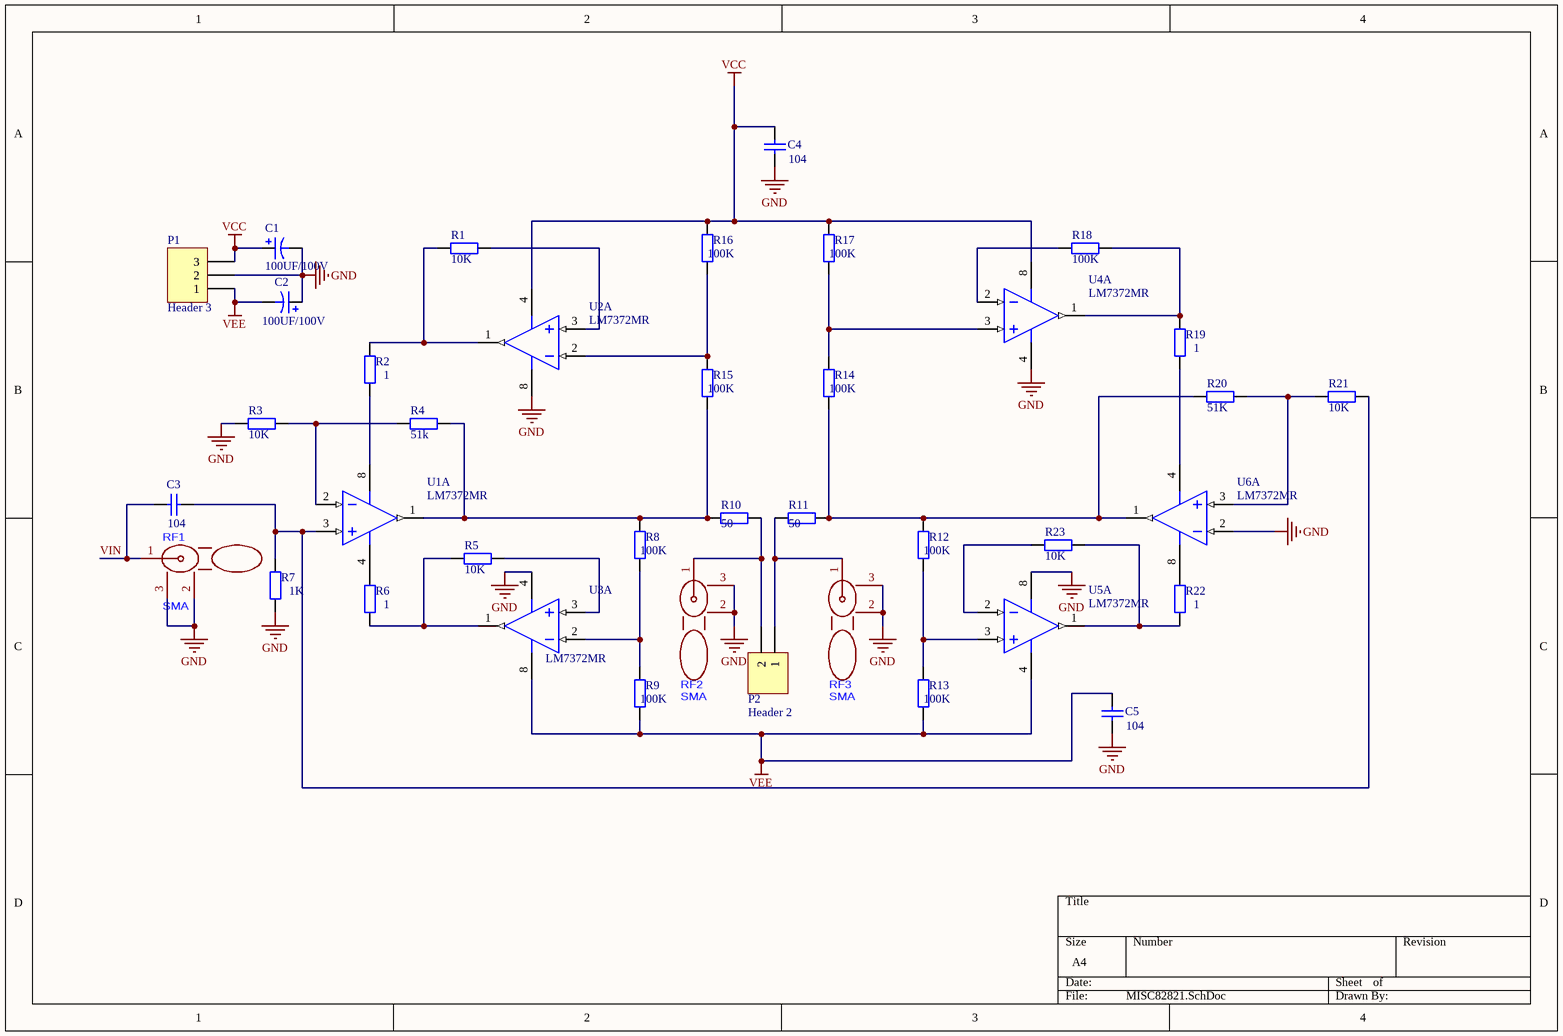
[diagram p0: MISC82821.SchDoc]
# Altium project MISC82821-15.PrjPcb
1 sheet, 39 parts. Net scope: global (net labels, ports and power ports of the same name join across sheets).
Board file: MISC82821.PcbDoc

## Sheet MISC82821.SchDoc
size A4

### Parts
C1  100UF/100V  [C0805]
C2  100UF/100V  [C0805]
C3  104  [C1206]
C4  104  [C1206]
C5  104  [C1206]
P1  Header 3  [HDR1X3]
P2  Header 2  [HDR1X2]
R1  10K  [AXIAL-0.4]
R2  1  [AXIAL-0.4]
R3  10K  [AXIAL-0.4]
R4  51k  [AXIAL-0.4]
R5  10K  [AXIAL-0.4]
R6  1  [AXIAL-0.4]
R7  1K  [AXIAL-0.4]
R8  100K  [AXIAL-0.4]
R9  100K  [AXIAL-0.4]
R10  50  [AXIAL-0.4]
R11  50  [AXIAL-0.4]
R12  100K  [AXIAL-0.4]
R13  100K  [AXIAL-0.4]
R14  100K  [AXIAL-0.4]
R15  100K  [AXIAL-0.4]
R16  100K  [AXIAL-0.4]
R17  100K  [AXIAL-0.4]
R18  100K  [AXIAL-0.4]
R19  1  [AXIAL-0.4]
R20  51K  [AXIAL-0.4]
R21  10K  [AXIAL-0.4]
R22  1  [AXIAL-0.4]
R23  10K  [AXIAL-0.4]
RF1  SMA  [SMA-SMD_HJ-SMA313]
RF2  SMA  [SMA-SMD_HJ-SMA313]
RF3  SMA  [SMA-SMD_HJ-SMA313]
U1  LM7372MR  [MRA08B_N]  (part A of 3)
U2  LM7372MR  [MRA08B_N]  (part A of 3)
U3  LM7372MR  [MRA08B_N]  (part A of 3)
U4  LM7372MR  [MRA08B_N]  (part A of 3)
U5  LM7372MR  [MRA08B_N]  (part A of 3)
U6  LM7372MR  [MRA08B_N]  (part A of 3)

### Nets
GND: C1.2 C2.1 C4.1 C5.1 P1.2 R3.1 R7.1 RF1.2 RF1.3 RF2.2 RF2.3 RF3.2 RF3.3 U2.8(V+) U3.4(V-) U4.4(V-) U5.8(V+) U6.2(INA-)
VCC: C1.1 C4.2 P1.3 R16.2 R17.2 U2.4(V-) U4.8(V+)
VEE: C2.2 C5.2 P1.1 R9.1 R13.1 U3.8(V+) U5.4(V-)
VIN: C3.2 RF1.1
NetC3_1: C3.1 R7.2 R21.2 U1.3(INA+)
NetP2_1: P2.1 R11.2 RF3.1
NetP2_2: P2.2 R10.1 RF2.1
NetR1_1: R1.1 R2.2 U2.1(OUTA)
NetR1_2: R1.2 U2.3(INA+)
NetR2_1: R2.1 U1.8(V+)
NetR3_2: R3.2 R4.1 U1.2(INA-)
NetR4_2: R4.2 R8.2 R10.2 R15.1 U1.1(OUTA)
NetR5_1: R5.1 R6.1 U3.1(OUTA)
NetR5_2: R5.2 U3.3(INA+)
NetR6_2: R6.2 U1.4(V-)
NetR8_1: R8.1 R9.2 U3.2(INA-)
NetR11_1: R11.1 R12.2 R14.1 R20.1 U6.1(OUTA)
NetR12_1: R12.1 R13.2 U5.3(INA+)
NetR14_2: R14.2 R17.1 U4.3(INA+)
NetR15_2: R15.2 R16.1 U2.2(INA-)
NetR18_1: R18.1 U4.2(INA-)
NetR18_2: R18.2 R19.2 U4.1(OUTA)
NetR19_1: R19.1 U6.4(V-)
NetR20_2: R20.2 R21.1 U6.3(INA+)
NetR22_1: R22.1 R23.2 U5.1(OUTA)
NetR22_2: R22.2 U6.8(V+)
NetR23_1: R23.1 U5.2(INA-)

### Library data of the parts
C1 C2 = Cap Pol3: Polarized Capacitor (Surface Mount); Published: 8-Jun-2000; LatestRevisionDate: 29-May-2009; LatestRevisionNote: IPC-7351 Footprint Added.; PackageReference: C0805; PackageDescription: Chip Capacitor; Value: 100UF/100V; Publisher: Altium Limited
C3-C5 = Cap Semi: Capacitor (Semiconductor SIM Model); Published: 8-Jun-2000; LatestRevisionDate: 29-May-2009; LatestRevisionNote: IPC-7351 Footprint Added.; PackageReference: C1206; PackageDescription: Chip Capacitor; Value: 104; Publisher: Altium Limited
P1 = Header 3: Header, 3-Pin; LatestRevisionDate: 17-Jul-2002; LatestRevisionNote: Re-released for DXP Platform.; Publisher: Altium Limited
P2 = Header 2: Header, 2-Pin; LatestRevisionDate: 17-Jul-2002; LatestRevisionNote: Re-released for DXP Platform.; Publisher: Altium Limited
R1-R17 R19-R23 = Res2: Resistor; Published: 8-Jun-2000; LatestRevisionDate: 17-Jul-2002; LatestRevisionNote: Re-released for DXP Platform.; PackageReference: AXIAL-0.4; PackageDescription: Axial Device, Thru-Hole; 2 Leads; 0.4 in Pin Spacing; Publisher: Altium Limited
  R1 R3 R5 R21 R23: Value: 10K
  R2 R6 R19 R22: Value: 1
  R4 R20: Value: 51K
  R7: Value: 1K
  R8 R9 R12-R17: Value: 100K
  R10 R11: Value: 50
R18 = Res2: Resistor; Value: 10K; Published: 8-Jun-2000; LatestRevisionDate: 17-Jul-2002; LatestRevisionNote: Re-released for DXP Platform.; PackageReference: AXIAL-0.4; PackageDescription: Axial Device, Thru-Hole; 2 Leads; 0.4 in Pin Spacing; Publisher: Altium Limited
RF1 RF3 = SMB: Antenna
RF2 = SMB: TI antenna
U1-U6 = LM7372MR: High Speed, High Output Current, Dual Operational Amplifier, 9-pin PSOP; Manufacturer: National Semiconductor; PackageTopMarking: NSXYTT*LM73*72MR; PowerWise: N; CompType: Amplifiers; Published: 4-Dec-2008; LatestRevisionDate: 13-Jan-2009; LatestRevisionNote: Sim Model Added.; DatasheetVersion: Jun-2008; PackageVersion: revB, Dec-2007; PackageReference: MRA08B; PackageDescription: Molded, PSOP .193 x .154 x .058in, 8 Lead, .050in Pitch, Large DAP; PartNumber: LM7372MR; RoHS: N; PinCount: 8; Code_JEDEC: MS-012-AA; ComponentLink1Description: LM7372 Datasheet; ComponentLink1URL: http://www.national.com/ds/LM/LM7372.pdf; ComponentLink2Description: LM7372 Web Page; ComponentLink2URL: http://www.national.com/pf/LM/LM7372.html; ComponentLink3Description: MRA08B Package Page; ComponentLink3URL: http://www.national.com/packaging/folders/mra08b.html; Publisher: Altium Limited